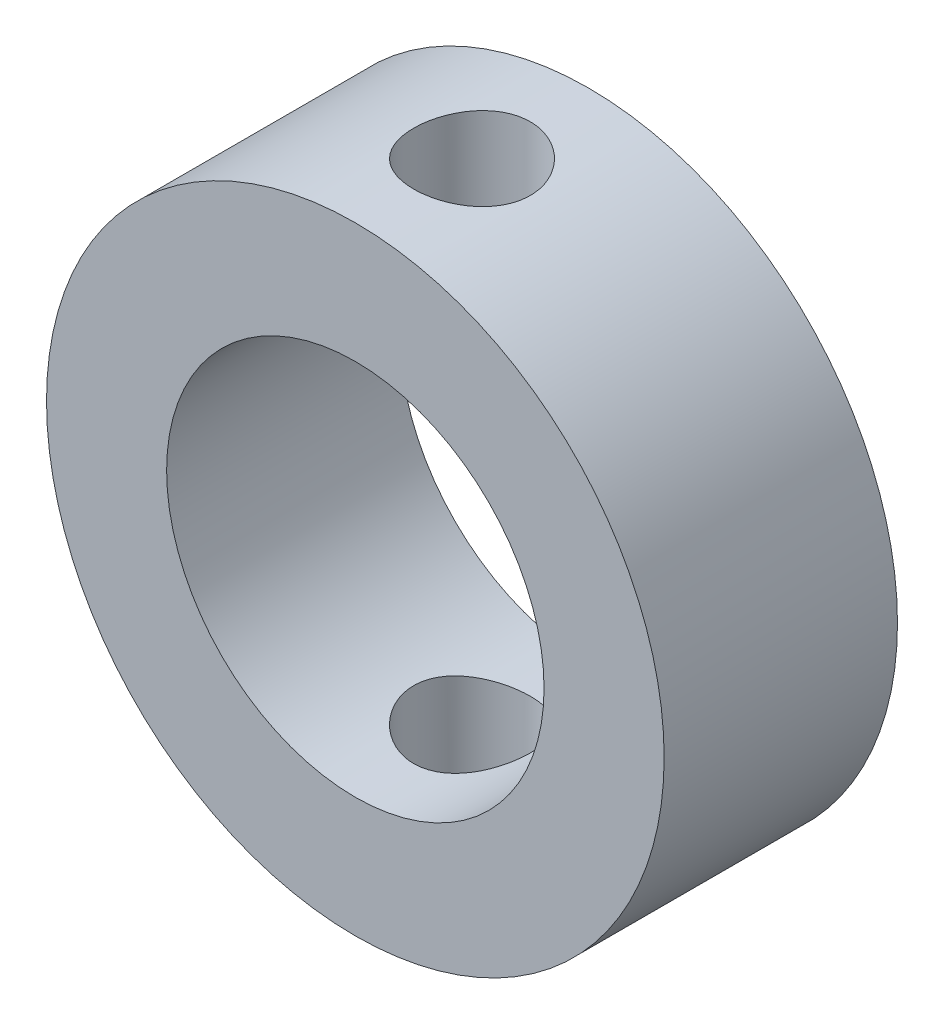
SolidWorks part; units mm, degrees
ref_plane "Front Plane" through (0, 0, 0) normal (0, 0, 1) x (1, 0, 0)
ref_plane "Top Plane" through (0, 0, 0) normal (0, 1, 0) x (1, 0, 0)
ref_plane "Right Plane" through (0, 0, 0) normal (1, 0, 0) x (0, 0, -1)
sketch "Sketch2" plane through (0, 0, 0) normal (0, 0, 1) x (1, 0, 0)
  circle A0 centre (0, 0) radius 27.5
  circle A1 centre (0, 0) radius 45
  dimension "D1" = 90
  dimension "D2" = 55
extrude "Boss-Extrude1" add sketch "Sketch2" along normal blind 34
sketch "Sketch3" plane through (0, 0, 0) normal (0, 1, 0) x (1, 0, 0)
  line L0 (-8.3512, -17) -> (73.5115, -17) construction
  circle A0 centre (0, -17) radius 8.5
  dimension "D2" = 17
  dimension "D1" = 17
extrude "Cut-Extrude1" cut sketch "Sketch3" against normal through all and the other way through all
